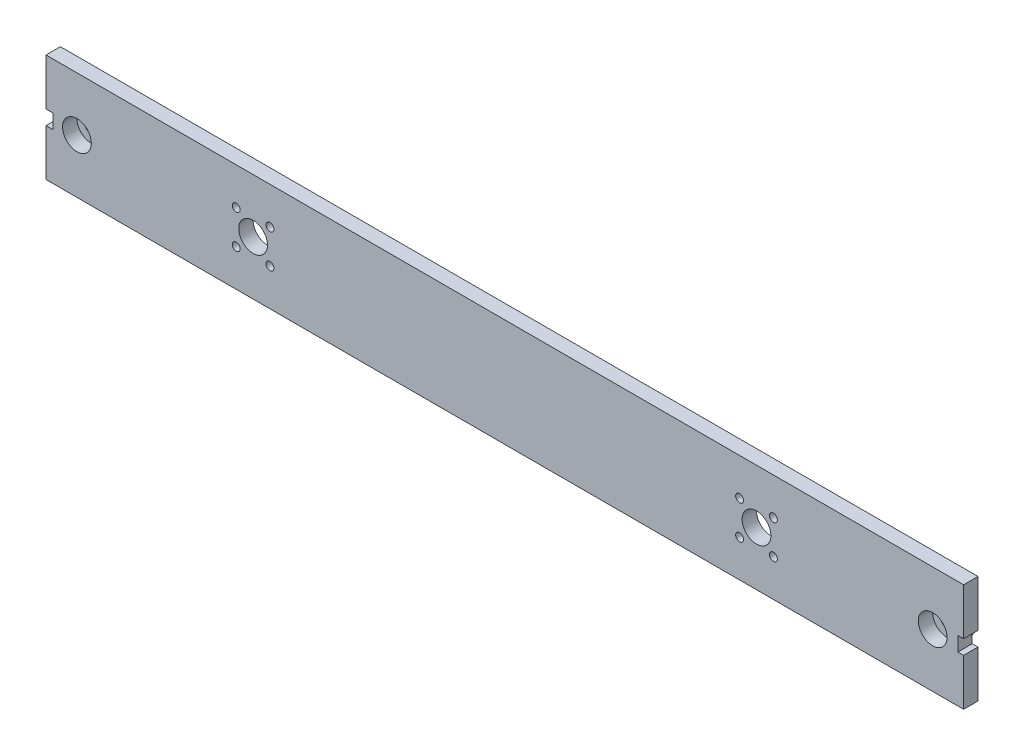
SolidWorks part; units mm, degrees
material "Q235"
ref_plane "Front Plane" through (0, 0, 0) normal (0, 0, 1) x (1, 0, 0)
ref_plane "Top Plane" through (0, 0, 0) normal (0, 1, 0) x (1, 0, 0)
ref_plane "Right Plane" through (0, 0, 0) normal (1, 0, 0) x (0, 0, -1)
sketch "Sketch1" plane through (0, 0, 0) normal (0, 0, 1) x (1, 0, 0)
  line L0 (0, 75) -> (1276, 75) construction
  line L1 (0, 0) -> (1276, 0)
  line L2 (0, 0) -> (0, 150)
  line L3 (0, 150) -> (1276, 150)
  line L4 (1276, 0) -> (1276, 150)
  line L5 (638, 150) -> (638, 0) construction
  line L6 (288, 75) -> (288, 150) construction
  circle A0 centre (288, 75) radius 20
  circle A1 centre (264.5, 98.5) radius 3.5
  circle A2 centre (311.5, 98.5) radius 3.5
  circle A3 centre (311.5, 51.5) radius 3.5
  circle A4 centre (264.5, 51.5) radius 3.5
  circle A5 centre (964.5, 51.5) radius 3.5
  circle A6 centre (1011.5, 51.5) radius 3.5
  circle A7 centre (988, 75) radius 20
  circle A8 centre (1011.5, 98.5) radius 3.5
  circle A9 centre (964.5, 98.5) radius 3.5
  dimension "D3" = 40
  dimension "D4" = 7
  dimension "D1" = 1276
  dimension "D2" = 150
  dimension "D5" = 350
  dimension "D6" = 47
  dimension "D7" = 23.5
  dimension "D8" = 47
  dimension "D10" = 23.5
extrude "Boss-Extrude1" add sketch "Sketch1" along normal blind 20
sketch "Sketch2" plane through (0, 0, 20) normal (0, 0, 1) x (1, 0, 0)
  circle A0 centre (264.5, 98.5) radius 5.5
  circle A1 centre (311.5, 98.5) radius 5.5
  circle A2 centre (311.5, 51.5) radius 5.5
  circle A3 centre (264.5, 51.5) radius 5.5
  circle A4 centre (964.5, 98.5) radius 5.5
  circle A5 centre (1011.5, 98.5) radius 5.5
  circle A6 centre (1011.5, 51.5) radius 5.5
  circle A7 centre (964.5, 51.5) radius 5.5
  dimension "D1" = 11
extrude "Cut-Extrude1" cut sketch "Sketch2" against normal blind 9
ref_plane "Plane1" through (638, 0, 0) normal (-1, 0, 0) x (0, 0, 1)
sketch "Sketch4" plane through (0, 0, 20) normal (0, 0, 1) x (1, 0, 0)
  line L0 (0, 150) -> (0, 0) construction
  line L1 (-10, 85) -> (10, 85)
  line L2 (-10, 85) -> (-10, 65)
  line L3 (-10, 65) -> (10, 65)
  line L4 (10, 85) -> (10, 65)
  line L5 (-10, 85) -> (10, 65) construction
  line L6 (-10, 65) -> (10, 85) construction
  line L7 (1276, 0) -> (1276, 150) construction
  line L8 (1268, 85) -> (1284, 85)
  line L9 (1268, 85) -> (1268, 65)
  line L10 (1268, 65) -> (1284, 65)
  line L11 (1284, 85) -> (1284, 65)
  line L12 (1268, 85) -> (1284, 65) construction
  line L13 (1268, 65) -> (1284, 85) construction
  point P0 (0, 75)
  point P7 (1276, 75)
  dimension "D1" = 16
  dimension "D2" = 20
  dimension "D3" = 20
  dimension "D4" = 20
extrude "Cut-Extrude2" cut sketch "Sketch4" against normal through all
sketch "Sketch5" plane through (0, 0, 20) normal (0, 0, 1) x (1, 0, 0)
  line L0 (638, 150) -> (638, 0) construction
  line L1 (1276, 150) -> (0, 150) construction
  line L2 (0, 0) -> (1276, 0) construction
  line L3 (10, 75) -> (43, 75) construction
  line L4 (10, 65) -> (10, 85) construction
  circle A0 centre (43, 75) radius 20
  circle A1 centre (1233, 75) radius 20
  dimension "D1" = 1190
  dimension "D2" = 40
extrude "Cut-Extrude3" cut sketch "Sketch5" against normal through all
sketch "Sketch6" plane through (0, 0, 0) normal (0, 0, 1) x (1, 0, 0)
  circle A0 centre (43, 75) radius 25
  circle A1 centre (43, 75) radius 9
  circle A2 centre (1233, 75) radius 25
  circle A3 centre (1233, 75) radius 9
  dimension "D1" = 50
  dimension "D2" = 18
extrude "Boss-Extrude2" add sketch "Sketch6" against normal blind 14 separate body
